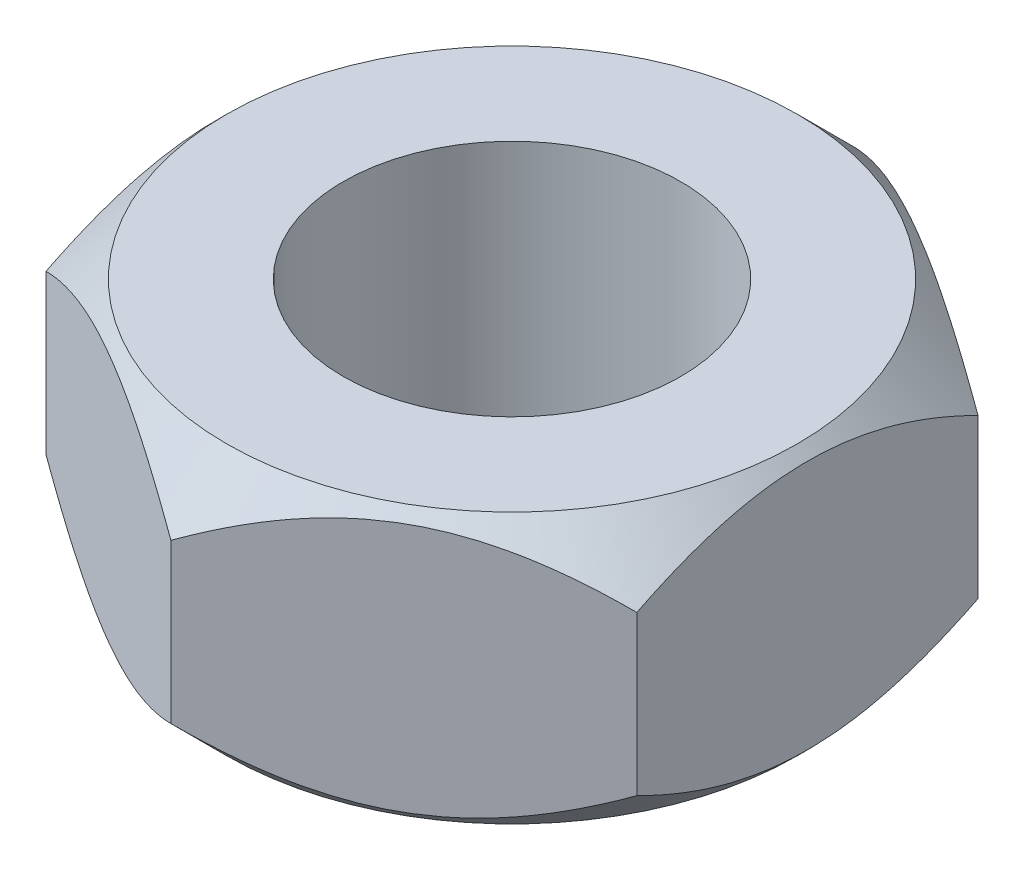
from build123d import *

# Parameters (mm, degrees)
BOSS_EXTRUDE1_DEPTH = 3.2
SKETCH8_R           = 2
CUT_EXTRUDE1_DEPTH  = 7.23083729


with BuildPart() as part:
    # Sketch1 → Boss-Extrude1 (new body)
    with BuildSketch(Plane(origin=(0, 0, 0), x_dir=(1, 0, 0), z_dir=(0, 1, 0))):
        Polygon((0, 4.041451884), (-3.5, 2.020725942), (-3.5, -2.020725942), (0, -4.041451884), (3.5, -2.020725942), (3.5, 2.020725942), align=None)
    extrude(amount=BOSS_EXTRUDE1_DEPTH)

    # Sketch3 → Cut-Revolve2 (revolve, cut)
    with BuildSketch(Plane(origin=(0, 0, 0), x_dir=(0.8660254037844417, 0, 0.4999999999999949), z_dir=(-0.4999999999999949, 0, 0.8660254037844417)), mode=Mode.PRIVATE) as cut_revolve2_sk:
        Polygon((4.041451884, 3.2), (4.041451884, 2.54), (3.381451884, 3.2), align=None)
        Polygon((4.041451884, 0), (4.041451884, 0.66), (3.381451884, 0), align=None)
    revolve(cut_revolve2_sk.sketch.rotate(Axis((0, -1.01584762, 0), (0, 1, 0)), 300), axis=Axis((0, -1.01584762, 0), (0, 1, 0)), mode=Mode.SUBTRACT)

    # Sketch8 → Cut-Extrude1 (cut, through all)
    with BuildSketch(Plane(origin=(0, 3.2, 0), x_dir=(1, 0, 0), z_dir=(0, 1, 0))):
        with Locations(Location((0, 0, 0), (0, 0, 270))):
            Circle(SKETCH8_R)
    extrude(amount=-CUT_EXTRUDE1_DEPTH, mode=Mode.SUBTRACT)


solid = part.part
